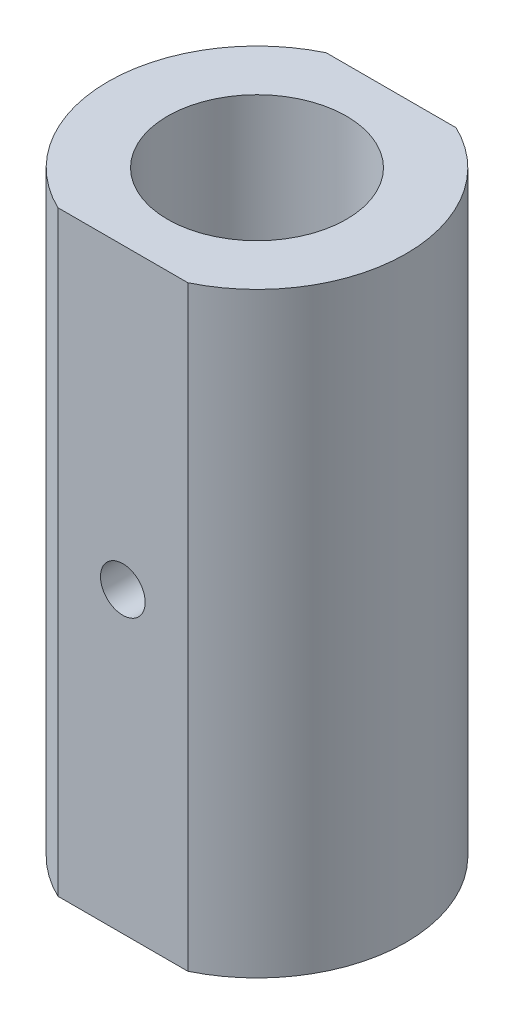
from build123d import *

# Parameters (mm, degrees)
SKETCH1_R           = 3
BOSS_EXTRUDE1_DEPTH = 20
SKETCH2_R           = 0.75
CUT_EXTRUDE1_DEPTH  = 20


with BuildPart() as part:
    # Sketch1 → Boss-Extrude1 (new body)
    with BuildSketch(Plane(origin=(0, 0, 0), x_dir=(1, 0, 0), z_dir=(0, 1, 0))):
        with BuildLine():
            Line((2.179449472, -4.5), (-2.179449472, -4.5))
            ThreePointArc((-2.179449472, -4.5), (-5, 0), (-2.179449472, 4.5))
            Line((-2.179449472, 4.5), (2.179449472, 4.5))
            ThreePointArc((2.179449472, 4.5), (5, 0), (2.179449472, -4.5))
        make_face()
        with Locations(Location((0, 0, 0), (0, 0, 270))):
            Circle(SKETCH1_R, mode=Mode.SUBTRACT)
    extrude(amount=BOSS_EXTRUDE1_DEPTH)

    # Sketch2 → Cut-Extrude1 (cut)
    with BuildSketch(Plane(origin=(0, 0, -4.5), x_dir=(-1, 0, 0), z_dir=(0, 0, -1))):
        with Locations((0, 10)):
            Circle(SKETCH2_R)
    extrude(amount=-CUT_EXTRUDE1_DEPTH, mode=Mode.SUBTRACT)


solid = part.part
